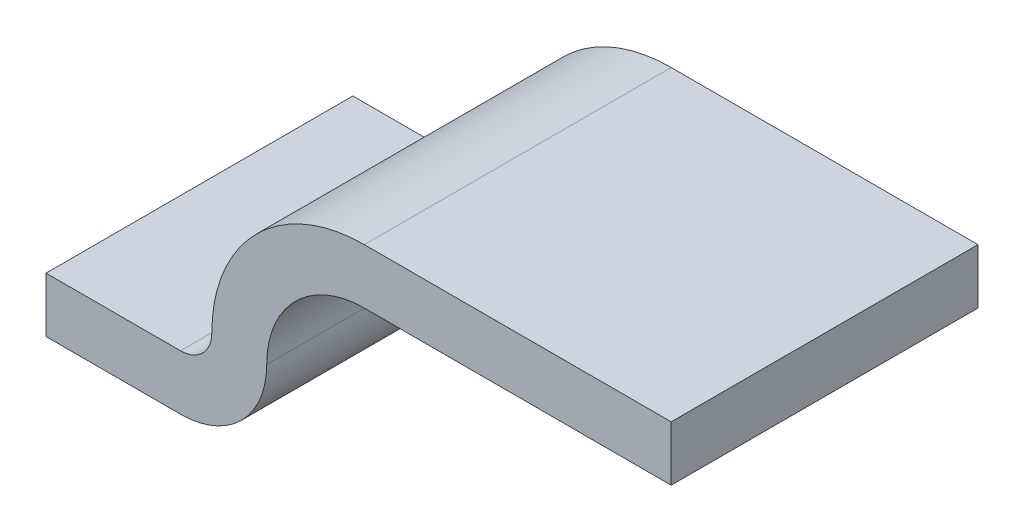
SolidWorks part; units mm, degrees
material "AISI 1020"
ref_plane "Front Plane" through (0, 0, 0) normal (0, 0, 1) x (1, 0, 0)
ref_plane "Top Plane" through (0, 0, 0) normal (0, 1, 0) x (1, 0, 0)
ref_plane "Right Plane" through (0, 0, 0) normal (1, 0, 0) x (0, 0, -1)
sketch "Sketch1" plane through (0, 0, 0) normal (0, 0, 1) x (1, 0, 0)
  line L0 (0, 11.112) -> (22.35, 11.112)
  line L1 (0, 7.112) -> (22.35, 7.112)
  line L2 (22.35, 11.112) -> (22.35, 7.112)
  line L3 (0, 0) -> (-22.2071, 0) construction
  line L4 (-13.392, 0) -> (-13.392, -8.724) construction
  line L5 (-13.392, -2.28) -> (-23.192, -2.28)
  line L6 (-13.392, -6.28) -> (-23.192, -6.28)
  line L7 (-23.192, -2.28) -> (-23.192, -6.28)
  arc A0 (0, 7.112) -> (-7.112, 0) centre (0, 0) ccw
  arc A1 (0, 11.112) -> (-11.112, 0) centre (0, 0) ccw
  arc A2 (-13.392, -2.28) -> (-11.112, 0) centre (-13.392, 0) ccw
  circle A4 centre (0, 0) radius 7.112 construction
  circle A5 centre (0, 0) radius 11.112 construction
  arc A6 (-13.392, -6.28) -> (-7.112, 0) centre (-13.392, 0) ccw
  point P1 (11.112, 0)
  point P12 (6.8012, 2.0793)
  dimension "D1" = 14.224
  dimension "D4" = 4.56
  dimension "D3" = 22.35
  dimension "D5" = 9.8
  dimension "D2" = 4
extrude "Boss-Extrude1" add sketch "Sketch1" along normal blind 22.352
